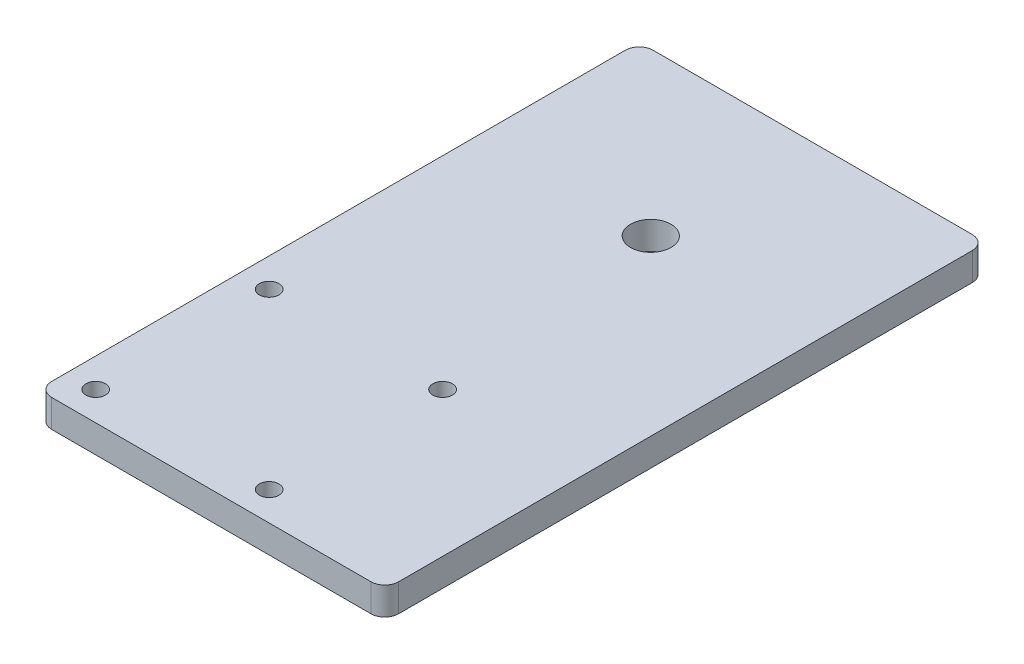
SolidWorks part; units mm, degrees
ref_plane "前视基准面" through (0, 0, 0) normal (0, 0, 1) x (1, 0, 0)
ref_plane "上视基准面" through (0, 0, 0) normal (0, 1, 0) x (1, 0, 0)
ref_plane "右视基准面" through (0, 0, 0) normal (1, 0, 0) x (0, 0, -1)
sketch "草图1" plane through (0, 0, 0) normal (0, 1, 0) x (1, 0, 0)
  line L1 (-75, 130) -> (75, 130)
  line L2 (-75, 130) -> (-75, -130)
  line L3 (-75, -130) -> (75, -130)
  line L4 (75, 130) -> (75, -130)
  line L5 (-75, 130) -> (75, -130) construction
  line L6 (-75, -130) -> (75, 130) construction
  point P0 (0, 0)
  dimension "D1" = 150
  dimension "D2" = 260
extrude "凸台-拉伸1" add sketch "草图1" along normal blind 12
fillet "圆角1" radius 6 4 edges at (75, 6, -130) (75, 6, 130) (-75, 6, 130) (-75, 6, -130)
hole_wizard "M20 螺纹孔1" positions "草图2" profile "草图3" tap size "M20" standard "GB"
sketch "草图2" plane through (0, 0, 0) normal (0, -1, 0) x (-1, 0, 0)
  line L0 (-69, 130) -> (69, 130) construction
  line L1 (-75, -124) -> (-75, 124) construction
  point P0 (0, 60)
  dimension "D1" = 70
  dimension "D2" = 75
sketch "草图3" plane through (0, 0, -60) normal (1, 0, 0) x (0, 0, -1)
  line L0 (0, 0) -> (0, 52.7575)
  line L1 (0, 52.7575) -> (8.75, 47.5)
  line L2 (8.75, 47.5) -> (8.75, 0)
  line L5 (8.75, 0) -> (0, 0)
  line L10 (0, 52.7575) -> (-8.75, 47.5) construction
  line L11 (0, -6.35) -> (0, 107.95) construction
  dimension "螺纹孔钻头直径" = 17.5
  dimension "螺纹孔钻头深度" = 47.5
  dimension "导头角度" = 118
cosmetic thread "孔螺蚊线1" parameters "D1"=12, "D2"=20
hole_wizard "M10 螺纹孔1" positions "草图4" profile "草图5" tap size "M10" standard "GB"
sketch "草图4" plane through (0, 0, 0) normal (0, -1, 0) x (-1, 0, 0)
  line L0 (75, 124) -> (75, -124) construction
  line L1 (69, -130) -> (-69, -130) construction
  point P0 (62.5, -117.5)
  point P2 (62.5, -42.5)
  point P4 (-12.5, -42.5)
  point P6 (-12.5, -117.5)
  dimension "D1" = 75
  dimension "D2" = 75
  dimension "D3" = 12.5
  dimension "D4" = 12.5
sketch "草图5" plane through (-62.5, 0, 117.5) normal (1, 0, 0) x (0, 0, -1)
  line L0 (0, 0) -> (0, 27.0537)
  line L1 (0, 27.0537) -> (4.25, 24.5)
  line L2 (4.25, 24.5) -> (4.25, 0)
  line L5 (4.25, 0) -> (0, 0)
  line L10 (0, 27.0537) -> (-4.25, 24.5) construction
  line L11 (0, -6.35) -> (0, 107.95) construction
  dimension "螺纹孔钻头直径" = 8.5
  dimension "螺纹孔钻头深度" = 24.5
  dimension "导头角度" = 118
cosmetic thread "孔螺蚊线2" parameters "D1"=12, "D2"=10
cosmetic thread "孔螺蚊线3" parameters "D1"=12, "D2"=10
cosmetic thread "孔螺蚊线4" parameters "D1"=12, "D2"=10
cosmetic thread "孔螺蚊线5" parameters "D1"=12, "D2"=10
